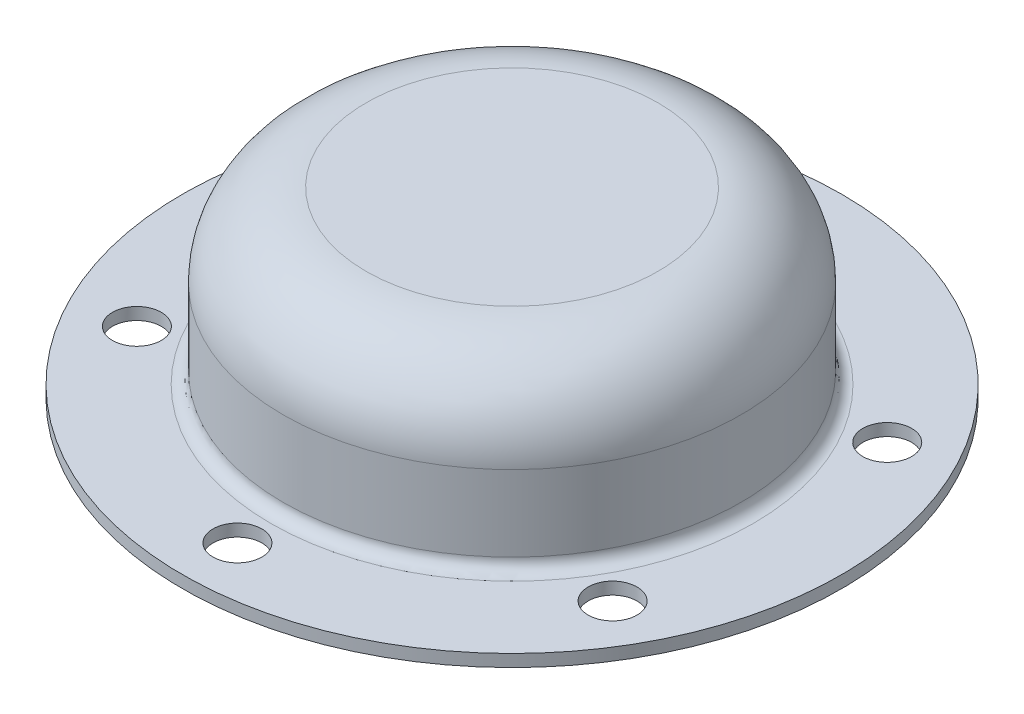
SolidWorks part; units mm, degrees
ref_plane "前视基准面" through (0, 0, 0) normal (0, 0, 1) x (1, 0, 0)
ref_plane "上视基准面" through (0, 0, 0) normal (0, 1, 0) x (1, 0, 0)
ref_plane "右视基准面" through (0, 0, 0) normal (1, 0, 0) x (0, 0, -1)
sketch "草图1" plane through (0, 0, 0) normal (0, 0, 1) x (1, 0, 0)
  line L3 (54, -13) -> (39.5, -13)
  line L4 (37.5, -11) -> (37.5, 1.4228)
  line L7 (54, -15) -> (37.5, -15)
  line L8 (35.5, -13) -> (35.5, 1.4228)
  line L9 (23.9228, 15) -> (0, 15)
  line L10 (0, 15) -> (0, 13)
  line L11 (0, 13) -> (23.9228, 13)
  line L12 (35.5, -15) -> (35.5, 1.4228) construction
  line L13 (54, -15) -> (35.5, -15) construction
  line L14 (54, -13) -> (37.5, -13) construction
  line L15 (37.5, -13) -> (37.5, 1.4228) construction
  line L16 (0, 0) -> (0, 13) construction
  line L17 (54, -15) -> (54, -13)
  arc A0 (37.5, 1.4228) -> (23.9228, 15) centre (23.9228, 1.4228) ccw
  arc A1 (35.5, 1.4228) -> (23.9228, 13) centre (23.9228, 1.4228) ccw
  arc A2 (35.5, -13) -> (37.5, -15) centre (37.5, -13) ccw
  arc A3 (39.5, -13) -> (37.5, -11) centre (39.5, -11) cw
  point P4 (0, 0)
  dimension "D5" = 2
  dimension "D1" = 37.5
  dimension "D2" = 54
  dimension "D3" = 2
  dimension "D4" = 30
revolve "旋转1" add sketch "草图1" angle 360 about L16
sketch "草图2" plane through (0, -13, 0) normal (0, 1, 0) x (1, 0, 0)
  circle A0 centre (0, 0) radius 45 construction
  circle A1 centre (0, 45) radius 4
  circle A2 centre (38.9711, 22.5) radius 4
  circle A3 centre (38.9711, -22.5) radius 4
  circle A4 centre (0, -45) radius 4
  circle A5 centre (-38.9711, -22.5) radius 4
  circle A6 centre (-38.9711, 22.5) radius 4
  dimension "D1" = 90
  dimension "D2" = 6
extrude "切除-拉伸1" cut sketch "草图2" against normal blind 10
